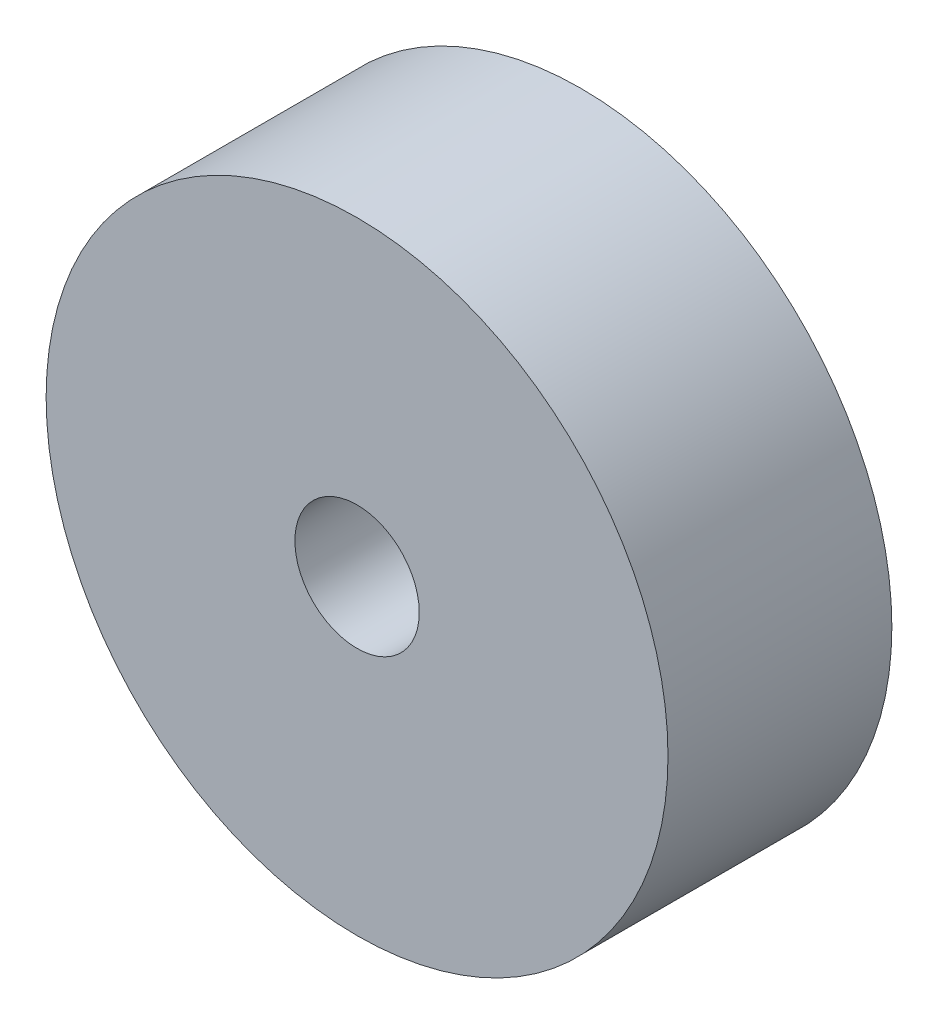
SolidWorks part; units mm, degrees
material "柔性聚氨酯泡沫体"
ref_plane "前视基准面" through (0, 0, 0) normal (0, 0, 1) x (1, 0, 0)
ref_plane "上视基准面" through (0, 0, 0) normal (0, 1, 0) x (1, 0, 0)
ref_plane "右视基准面" through (0, 0, 0) normal (1, 0, 0) x (0, 0, -1)
other "Configuration Table"
sketch "草图1" plane through (0, 0, 0) normal (0, 1, 0) x (1, 0, 0)
  line L0 (0, -129.0631) -> (0, 6324.094) construction
  line L1 (-2.5, 0) -> (-12.5, 0)
  line L2 (-12.5, 0) -> (-12.5, 9)
  line L3 (-12.5, 9) -> (-2.5, 9)
  line L4 (-2.5, 9) -> (-2.5, 0)
  dimension "D1" = 5
  dimension "D2" = 25
  dimension "D3" = 9
revolve "旋转1" add sketch "草图1" angle 360 about L0
